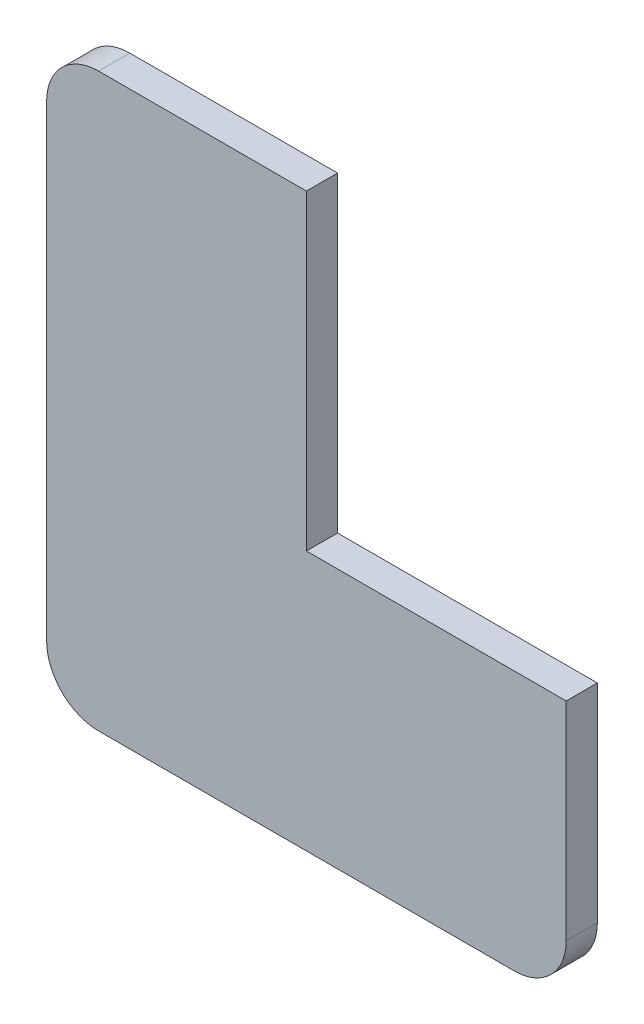
SolidWorks part; units mm, degrees
ref_plane "Front Plane" through (0, 0, 0) normal (0, 0, 1) x (1, 0, 0)
ref_plane "Top Plane" through (0, 0, 0) normal (0, 1, 0) x (1, 0, 0)
ref_plane "Right Plane" through (0, 0, 0) normal (1, 0, 0) x (0, 0, -1)
sketch "Sketch1" plane through (0, 0, 0) normal (0, 0, 1) x (1, 0, 0)
  line L0 (-385, 217.5147) -> (-385, 6) construction
  line L1 (-360, -3) -> (-385, -3)
  line L2 (-360, -3) -> (-360, -23)
  line L3 (-365, -28) -> (-405, -28)
  line L4 (-410, -3) -> (-410, -23)
  line L6 (-385, 27) -> (-405, 27)
  line L7 (-385, 27) -> (-385, -3)
  line L9 (-410, 22) -> (-410, -3)
  arc A0 (-360, -23) -> (-365, -28) centre (-365, -23) cw
  arc A1 (-405, -28) -> (-410, -23) centre (-405, -23) cw
  arc A2 (-405, 27) -> (-410, 22) centre (-405, 22) ccw
  point P12 (-360, -28)
  point P15 (-410, -28)
  dimension "D4" = 5
  dimension "D1" = 50
  dimension "D2" = 25
  dimension "D3" = 30
extrude "Boss-Extrude1" add sketch "Sketch1" along normal blind 3
